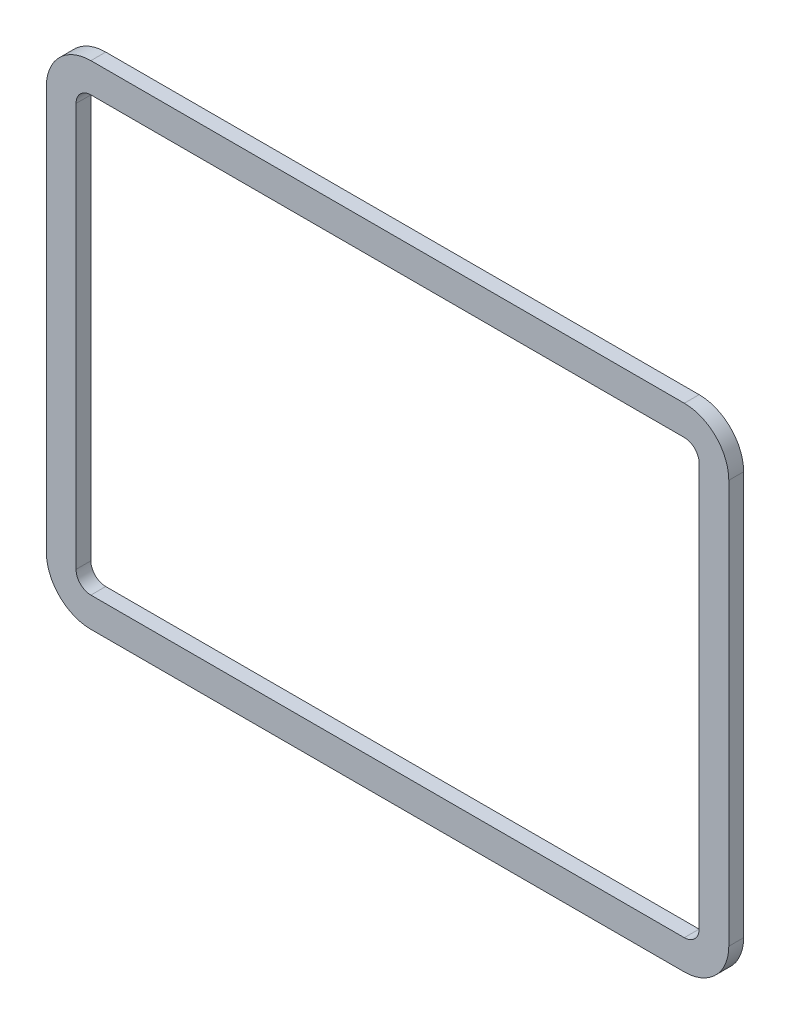
SolidWorks part; units mm, degrees
material "Plain Carbon Steel"
ref_plane "Front Plane" through (0, 0, 0) normal (0, 0, 1) x (1, 0, 0)
ref_plane "Top Plane" through (0, 0, 0) normal (0, 1, 0) x (1, 0, 0)
ref_plane "Right Plane" through (0, 0, 0) normal (1, 0, 0) x (0, 0, -1)
sketch "Sketch1" plane through (0, 0, 0) normal (0, 0, 1) x (1, 0, 0)
  line L0 (0, -3303.8058) -> (0, 161886.4829) construction
  line L1 (-3303.8058, 0) -> (161886.4829, 0) construction
  line L2 (-105, 73) -> (105, 73)
  line L3 (-115, 83) -> (115, 83)
  line L4 (-115, 83) -> (-115, -83)
  line L5 (-115, -83) -> (115, -83)
  line L6 (115, 83) -> (115, -83)
  line L7 (105, 73) -> (105, -73)
  line L8 (-105, -73) -> (105, -73)
  line L9 (-105, 73) -> (-105, -73)
  dimension "D1" = 230
  dimension "D2" = 166
  dimension "D3" = 10
extrude "Boss-Extrude1" add sketch "Sketch1" along normal blind 5
fillet "Fillet1" radius 5 4 edges at (-105, 73, 2.5) (105, 73, 2.5) (105, -73, 2.5) (-105, -73, 2.5)
fillet "Fillet2" radius 15 4 edges at (115, -83, 2.5) (115, 83, 2.5) (-115, 83, 2.5) (-115, -83, 2.5)
